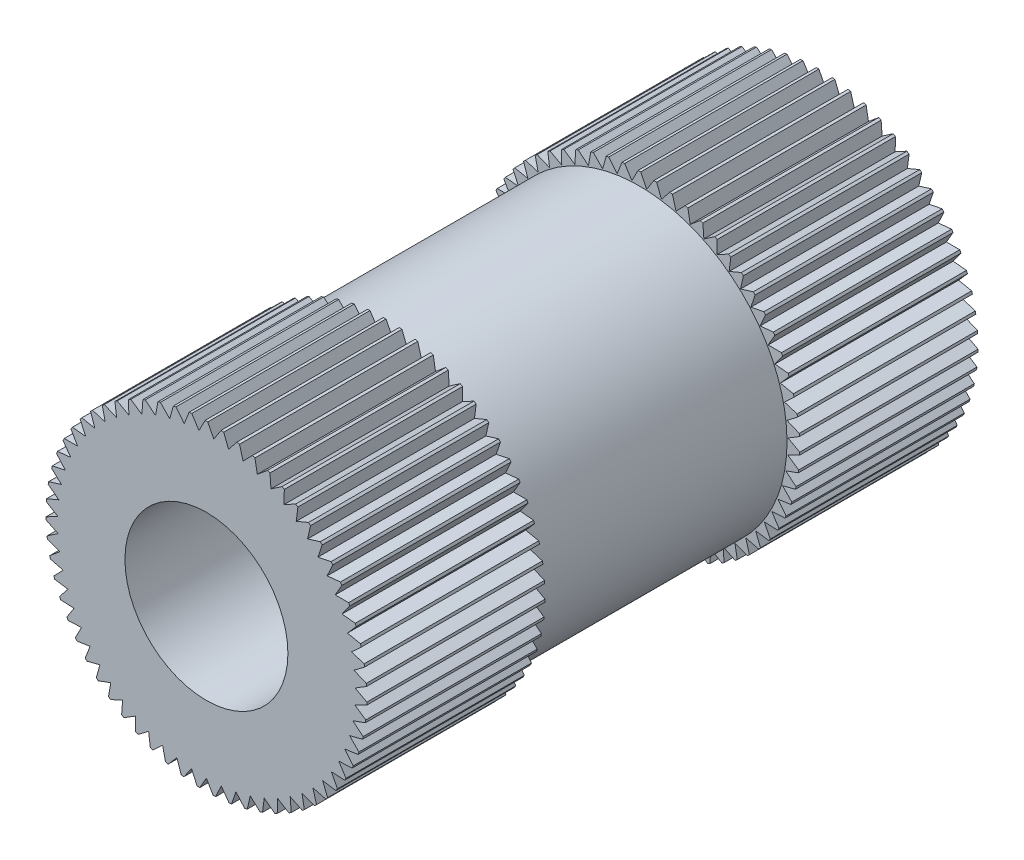
from build123d import *

# Parameters (mm, degrees)
SKETCH_1_R               = 3.15
SKETCH_1_R_2             = 1.6
EXTRUDE_1_DEPTH          = 6
CUT_EXTRUDE_1_DEPTH      = 12
PATTERN_CIRCULAR_1_COUNT = 63
SKETCH_3_R               = 3.663083808
SKETCH_3_R_2             = 2.9
CUT_EXTRUDE_2_DEPTH      = 2.5


with BuildPart() as part:
    # 草图1 → 凸台-拉伸1 (new, symmetric)
    with BuildSketch(Plane.XY):
        Circle(SKETCH_1_R)
        Circle(SKETCH_1_R_2, mode=Mode.SUBTRACT)
    extrude(amount=EXTRUDE_1_DEPTH, both=True)

    # 草图2 → 切除-拉伸1 (cut)
    with BuildSketch(Plane.XY.offset(6)):
        Polygon((0, -2.920487935), (-0.348301486, -3.523763805), (0.348301486, -3.523763805), align=None)
    cut_extrude_1 = extrude(amount=-CUT_EXTRUDE_1_DEPTH, mode=Mode.SUBTRACT)

    # 阵列(圆周)1: 切除-拉伸1 ×63 about axis
    pattern_circular_1_axis = Axis((0, 0, 0), (0, 0, 1))
    for i in range(1, PATTERN_CIRCULAR_1_COUNT):
        add(cut_extrude_1.rotate(pattern_circular_1_axis, i * 360 / PATTERN_CIRCULAR_1_COUNT), mode=Mode.SUBTRACT)

    # 草图3 → 切除-拉伸2 (cut, symmetric)
    with BuildSketch(Plane.XY):
        Circle(SKETCH_3_R)
        Circle(SKETCH_3_R_2, mode=Mode.SUBTRACT)
    extrude(amount=CUT_EXTRUDE_2_DEPTH, both=True, mode=Mode.SUBTRACT)


solid = part.part
